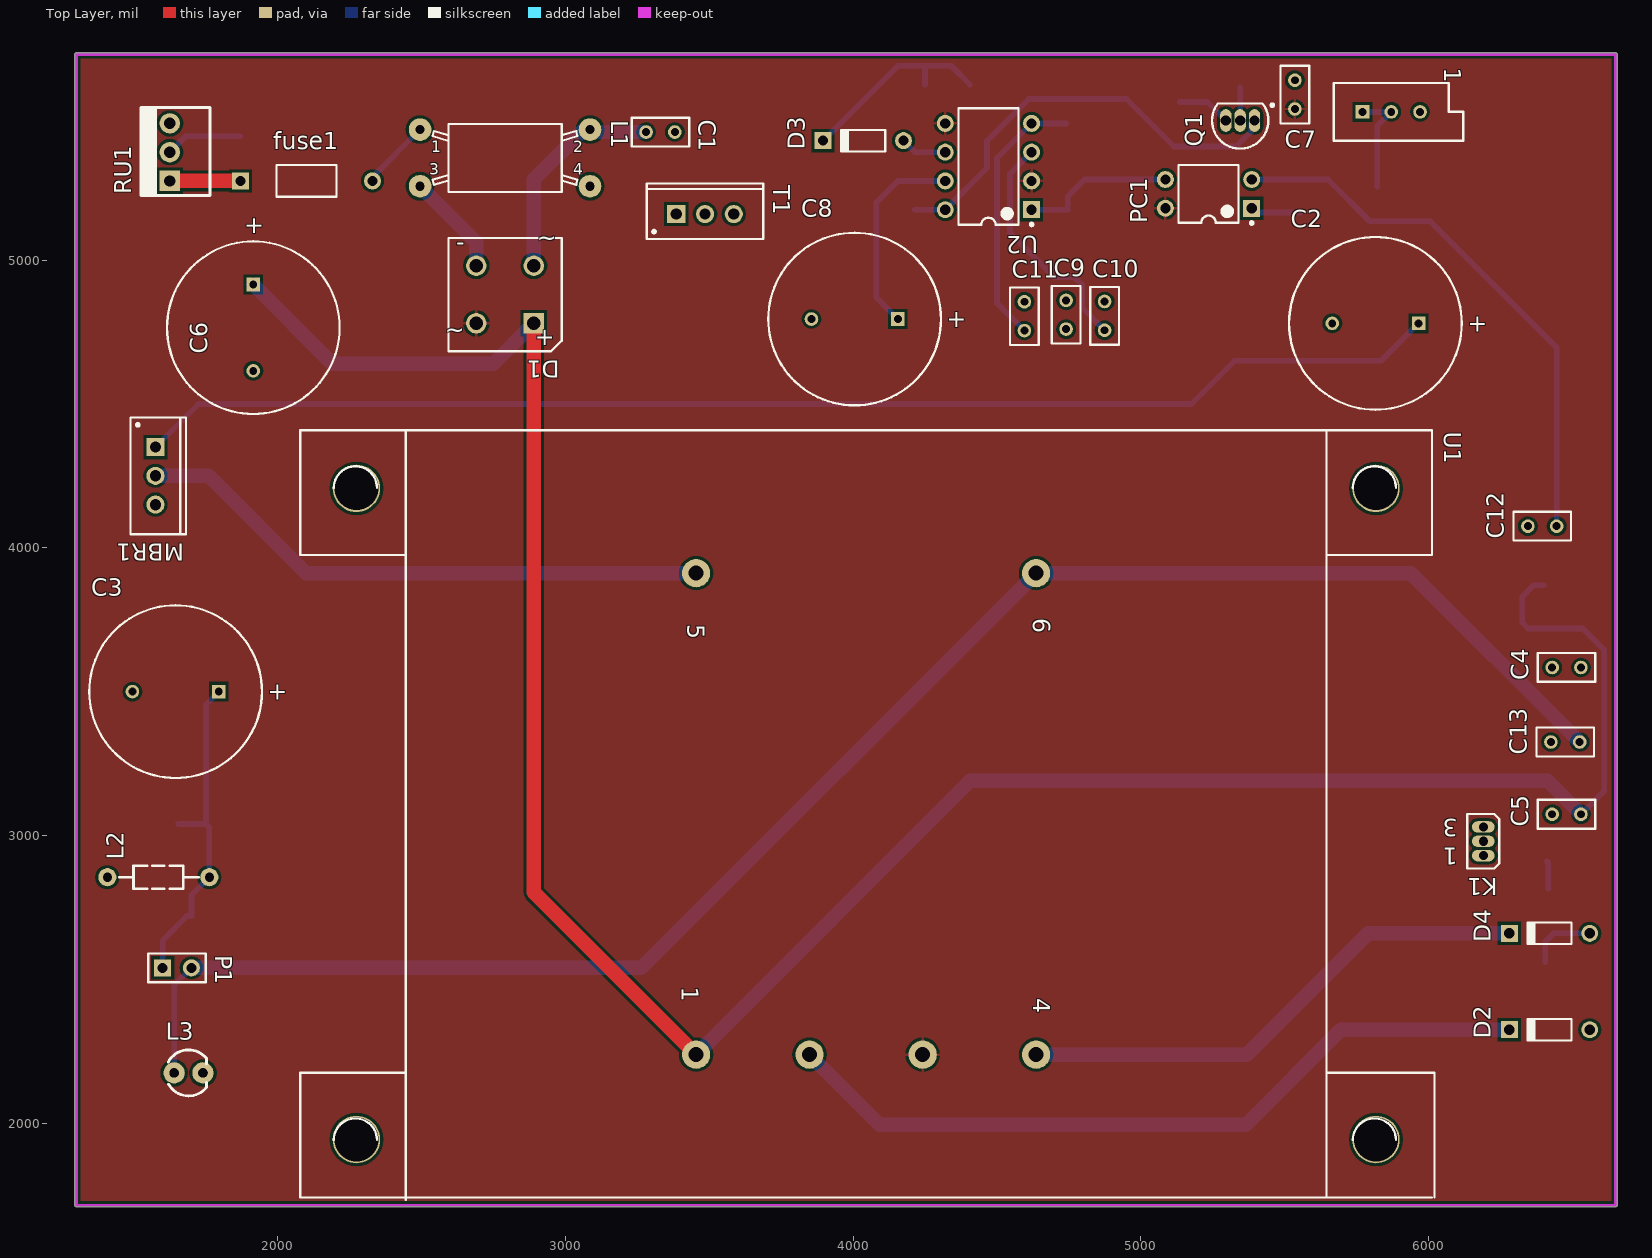
[diagram p0: Top Layer view]
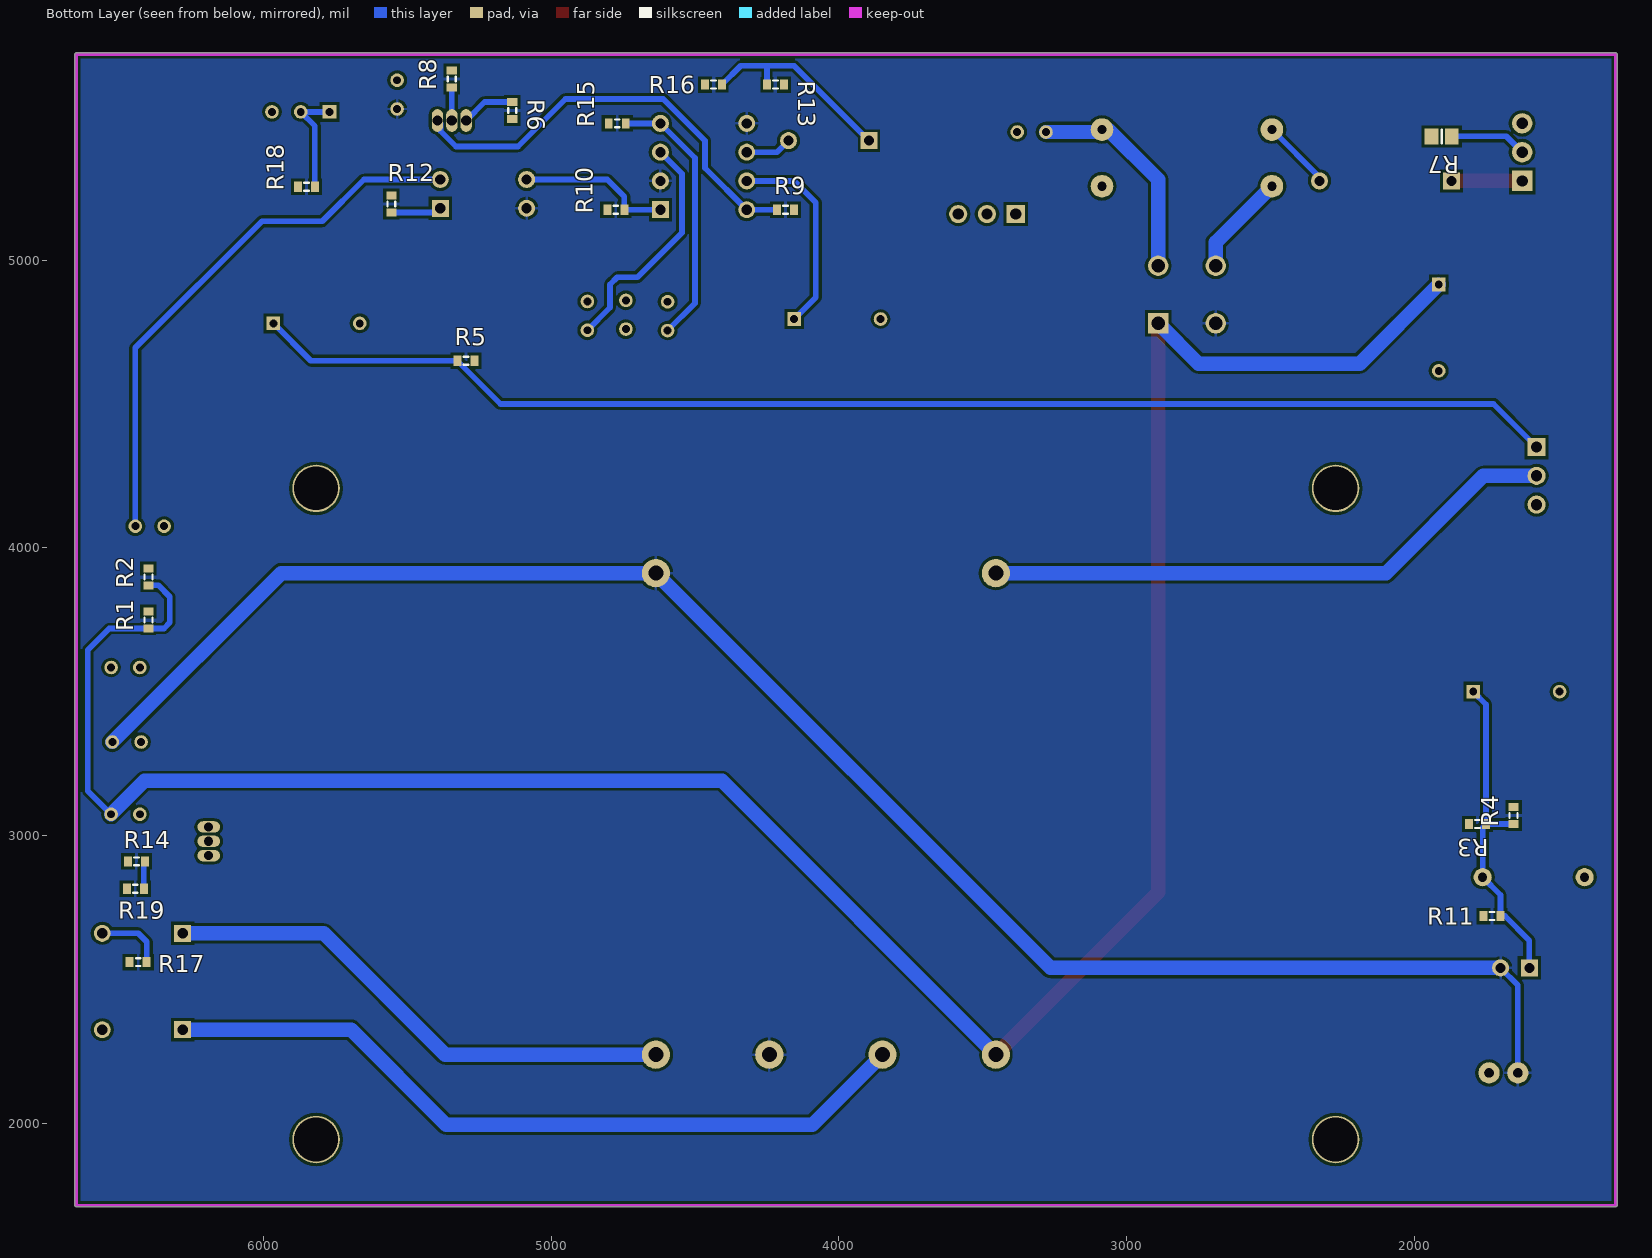
[diagram p1: Bottom Layer view, seen from below]
# Altium PCB MISC82118.PcbDoc
Units mil, origin at the board's own origin, x right, y up, seen from the top; angles counter-clockwise.
Board outline 5360.03 x 4010.03 mil, 2 copper layers (Top Layer, Bottom Layer); 50 components, 32 nets, 126 pads, 0 vias.

## Layer stack, top to bottom (the 12.6 mil dielectric is the usual default, probably not edited)
Top Solder: solder mask 0.4, Solder Resist, Dk 3.5
Top Layer: signal copper 1.4
Dielectric 1: dielectric 12.6, FR-4, Dk 4.8
Bottom Layer: signal copper 1.4
Bottom Solder: solder mask 0.4, Solder Resist, Dk 3.5

## Board outline
1300,1709.98 cw(c1300,1715) 1294.98,1715 1294.98,5715 cw(c1300,5715) 1300,5720.02 6650,5720.02 cw(c6650,5715) 6655.02,5715 6655.02,1715 cw(c6650,1715) 6650,1709.98

## Design rules (kind name [scope] priority, off if disabled: settings)
Clearance [All] p1: gap=10
MinimumSolderMaskSliver [All] p1: minsoldermaskwidth=0
PolygonConnect [All] p1: connectstyle=Relief reliefconductorwidth=10 reliefentries=4 polygonreliefangle="90 Angle" airgapwidth=10
RoutingVias [All] p1: holewidth=28 width=50 viastyle="Through Hole" minholewidth=28 minwidth=50 maxholewidth=28 maxwidth=50
SilkToSilkClearance [All] p1: silktosilkclearance=0
SilkToSolderMaskClearance [IsPad] p1: minsilkscreentomaskgap=0 clearancetoexposedcopper=TRUE
SolderMaskExpansion [All] p1: expansion=4
Width [All] p1: maxlimit=70 minlimit=10 preferedwidth=10
27 further rules are at their usual default settings.

## Components (designator, comment, footprint, x,y, rotation, side; value= is the part's Value field where it differs from the comment)
1 "" VR5 5870,5515 r0 top
C1 "0.1u 275V" RAD-0.1 3330,5445 r0 top
C2 "35V 1000U" RB7.6-15 5815,4780 r0 top
C3 "35V 1000U" RB7.6-15 1645,3500 r0 top
C4 "2KV 103" RAD-0.1 6479.33,3583.94 r180 top
C5 "222/2KV" RAD-0.1 6479.33,3073.94 r180 top
C6 "400V  82uF" RB7.6-15 1915,4765 r90 top
C7 "104" RAD-0.1 5535,5575 r90 top
C8 "35V100U" RB7.6-15 4005,4795 r0 top
C9 "225" RAD-0.1 4740,4810 r90 top
C10 "471" RAD-0.1 4873.77,4806.06 r90 top
C11 "222" RAD-0.1 4595,4805 r90 top
C12 "104" RAD-0.1 6395,4075 r180 top
C13 "104" RAD-0.1 6475,3325 r180 top
D1 "1N4007*4" D-38 2790,4880 r180 top
D2 "FR107" DO-35 6420,2325 r180 top
D3 "IN4148" DO-35 4035,5415 r180 top
D4 "FR107" DO-35 6420,2660 r180 top
fuse1 "" PIN-W2/E2.8 2100,5275 r0 top
K1 "20N60" E3 6190,2980 r180 top
L1 "Filter" TRANS 2790,5355 r0 top
L2 "100UH" AL0204 1585,2855 r180 top
L3 "LED" LED3MM 1690,2175 r0 top
MBR1 "" TO-262-AA 1575,4250 r270 top
P1 "Output" HDR1X2 1600,2540 r0 top
PC1 "*" DIP-4 5235,5230 r180 top
Q1 "S8550" TO-92A 5345,5485 r90 top
R1 "2W 150K" J1-0603 6399.33,3748.94 r90 bottom
R2 "2W 200K" J1-0603 6399.33,3898.94 r90 bottom
R3 "2W 330" J1-0603 1780,3040 r0 bottom
R4 "2K2" J1-0603 1655,3070 r90 bottom
R5 "10/1W" J1-0603 5295.47,4650 r180 bottom
R6 "68k" J1-0603 5135,5519.53 r270 bottom
R7 "NTC 5D-11" 6-0805_N 1904.57,5430 r0 bottom
R8 "4K1" J1-0603 5345,5629.53 r90 bottom
R9 "680" J1-0603 4185,5175 r180 bottom
R10 "4K1" J1-0603 4775,5175 r0 bottom
R11 "20K" J1-0603 1730,2720 r0 bottom
R12 "470" J1-0603 5555,5195 r90 bottom
R13 "15" J1-0603 4220.47,5610 r180 bottom
R14 "470" J1-0603 6440.47,2910 r0 bottom
R15 "18K" J1-0603 4770,5475 r0 bottom
R16 "1K" J1-0603 4435,5610 r0 bottom
R17 "1W 10" J1-0603 6435,2560 r0 bottom
R18 "2K2" J1-0603 5850.47,5255 r0 bottom
R19 "2W 0.62" J1-0603 6445,2815 r0 bottom
RU1 "*" KF2510-3P 1625,5275 r90 top
T1 "TL431" TO-262-AA 3485,5160 r0 top
U1 "Transformer 1" TRF_6 4045,3075 r270 top
U2 "UC3842" DIP-8 4470,5325 r180 top

## Footprints (in the part's own frame and the unit in brackets; to place one, negate y for a bottom-side part, rotate by r counter-clockwise, add the part's x,y. Pads: shape width x height; smd on the part's side, far side on the other; paste and mask are expansions set on the pad)
6-0805_N [mm] "Chip Resistor, Body 2.0x1.2mm, IPC Medium Density"
  rect 1.2x1.4 smd: 1(-0.9,0) 2(0.9,0)
  silkscreen extent 0,-0.6 0,0.6, body extent -1.07,-0.7 1.07,0.7, height 0.7
AL0204 [mm] "9*2*4mm（脚距，直径，长度）"
  round 1.6 hole 0.8: 1(-4.5,0) 2(4.5,0)
  silkscreen extent -3.56,-1.02 3.43,1.02, body extent -4.75,-1.02 4.75,1.02, height 2.07
D-38 [mm] "Bridge Rectifier; 4 Terminals; Body 9.4 x 9.4 mm (typ); Pitch 5.08 mm"
  rect 1.8x1.8 hole 1.2: 1(-2.54,2.54)
  round 1.8 hole 1.2: 2(-2.54,-2.54) 3(2.54,-2.54) 4(2.54,2.54)
  silkscreen extent -5,-5 5,5, body extent -5,-5 5,5, height 9.91
DIP-4 [mm] "DIP; 4 Leads; Row Spacing 7.62 mm; Pitch 2.54 mm"
  rect 1.5x1.5 hole 0.9: 1(-3.81,1.27)
  round 1.5 hole 0.9: 2(-3.81,-1.27) 3(3.81,-1.27) 4(3.81,1.27)
  silkscreen extent -3.94,-2.55 2.65,2.69, body extent -3.15,-2.5 3.15,2.5, height 5.6
DIP-8 [mm] "DIP; 8 Leads; Row Spacing 7.62 mm; Pitch 2.54 mm"
  rect 1.5x1.5 hole 0.9: 1(-3.81,3.81)
  round 1.5 hole 0.9: 2(-3.81,1.27) 3(-3.81,-1.27) 4(-3.81,-3.81) 5(3.81,-3.81) 6(3.81,-1.27) 7(3.81,1.27) 8(3.81,3.81)
  silkscreen extent -3.94,-5.15 2.65,5.23, body extent -3.6,-5.15 3.6,5.15, height 5.08
DO-35 [mm] "Diode, Axial; Body 3.8 x 1.9 mm (LxDia. max), Lead Dia. 0.53 mm (max)"
  round 1.5 hole 0.9: 1(-3.55,0)
  rect 1.5x1.5 hole 0.9: 2(3.55,0)
  silkscreen extent -1.95,-0.95 2.05,0.95
E3 [mm] "TO, Flat Index; 3 In-Line, Axial Leads; Body Dia. 4.6mm; Lead Dia. 0.5 mm (max)"
  oval 2x1 hole 0.8: 1(0,1.27) 2(0,0) 3(0,-1.27)
  silkscreen extent -1.41,-2.41 1.41,2.41
HDR1X2 [mm] "Connector; Header; 2 Position"
  rect 1.5x1.5 hole 0.9: 1(0,0)
  round 1.5 hole 0.9: 2(2.54,0)
  silkscreen extent -1.27,-1.27 3.81,1.27
J1-0603 [mm] "Chip Resistor, Body 1.6x0.8mm, IPC High Density"
  rect 0.7x0.9 smd: 1(-0.75,0) 2(0.75,0)
  silkscreen extent -0.2,-0.35 0.2,0.35, body extent -0.85,-0.48 0.85,0.48, height 0.9
KF2510-3P [mm]
  rect 1.8x1.8 hole 1: 1(0,0)
  round 1.8 hole 1: 2(2.54,0) 3(5.08,0)
  silkscreen extent -1.27,-3.56 6.48,2.54, body extent -1.27,-3.59 6.35,2.32, height 11.05
LED3MM [mil]
  round 74 hole 32 slot 32.2 at 0 deg paste+0 mask+2: 1(-50,0) 2(50,0)
  silkscreen extent -71,-80 62,80
PIN-W2/E2.8 [mm] "Thru-Hole; 2 Leads"
  rect 1.5x1.5 hole 0.9: 1(-5.825,0)
  round 1.5 hole 0.9: 2(5.825,0)
  silkscreen extent -2.65,-1.4 2.65,1.4
RAD-0.1 [mm] "Radial Cap, Thru-Hole; 2 Leads; 0.1 in Pin Spacing"
  round 1.2 hole 0.7: 1(-1.27,0) 2(1.27,0)
  silkscreen extent -2.54,-1.27 2.54,1.27
RB7.6-15 [mm] "Polarized Capacitor (Radial); 2 Leads"
  rect 1.2x1.2 hole 0.7: 1(3.81,0)
  round 1.2 hole 0.7: 2(-3.81,0)
  silkscreen extent -7.62,-7.62 7.62,7.62
TO-92A [mm] "TO, Flat Index; 3 In-Line, Axial Leads; Body Dia. 4.5mm; Leads 0.51 x 0.48 mm (max)"
  oval 2x1 hole 0.9: 1(0,-1.27) 2(0,0) 3(0,1.27)
  silkscreen extent -2.48,-2.96 1.5,2.48, body extent -2.48,-2.5 1.5,2.5, height 6.86
TO-262-AA [mm] "TO, Thru-Hole, Vertical, Heatsink Mounted; 3 In-Line Leads; Pitch 2.54 mm"
  rect 1.6x1.6 hole 1: 1(-2.54,0)
  round 1.6 hole 1: 2(0,0) 3(2.54,0)
  silkscreen extent -5.15,-2.2 5.15,2.7, body extent -5.2,-2.25 5.2,2.75, height 19.7
TRANS [mm] "Transformer; 4 Leads"
  round 2 hole 0.8: 1(-7.5,2.5) 2(7.5,2.5) 3(-7.5,-2.5) 4(7.5,-2.5)
  silkscreen extent -6.4,-3 6.4,3
TRF_6 [mil] "Transformer; 6 Leads"
  round 98 hole 52: 1(836.67,-590.83) 2(836.67,-196.67) 3(836.67,196.67) 4(836.67,590.83) 5(-836.67,-590.83) 6(-836.67,590.83)
  round 165 hole 152: MH1(-1131.67,-1771.67) MH2(1131.67,-1771.67) MH3(1131.67,1771.67) MH4(-1131.67,1771.67)
  silkscreen extent -1333,-1967 1342,1975
VR5 [mm] "Thru-Hole; 3 Leads"
  rect 1.2x1.2 hole 0.7: 1(-2.54,0)
  round 1.2 hole 0.7: 2(0,0) 3(2.54,0)
  silkscreen extent -5.08,-2.54 6.35,2.54

## Part data
1: library part 三角电位器
C1 C4 C5 C7 C9 C10 C11 C12 C13: library part 电容
C2 C3 C6 C8: library part 电解电容1
D1: library part BRIDGE1, "Diode Bridge"
D2 D4: library part 肖特基二极管
D3: library part 二极管
fuse1: library part 保险丝
K1: library part N-MOS
L1: library part 滤波器
L2: library part 电感
L3: library part 发光二极管
MBR1: library part 肖特基二极管2
P1: library part "Header 2", "Header, 2-Pin"
PC1: library part 光电耦合器
Q1: library part 2N3906, "PNP General Purpose Amplifier"
R1 R2 R3 R4 R5 R6 R7 R8 R9 R10 R11 R12 R13 R14 R15 R16 R17 R18 R19: library part 电阻
RU1: library part 接线端子3
U1: library part 变压器1

## Nets (pads, with @x,y where several pads share a name; then routed paths per layer and width w, separated by ;. In a path a pad name is that pad's centre, name@x,y a point inside that pad or via, vN(x,y) a via of type N, cw(c..) or ccw(c..) an arc to the next point about the centre after c; other vN are vias at no path point)
GND: C7.1 C13.1 D1.4 L3.1 P1.2 PC1.4 U1.3 U1.6 U2.2 U2.5 | length 6026
  Bottom Layer w20: L3.1 1640,2480 P1.2
  Bottom Layer w50: P1.2 3264.17,2540 U1.6 5938.33,3911.67 C13.1
Net1_1: 1.1 1.2 R18.1 | length 380.3
  Bottom Layer w20: 1.1 1.2 5820.94,5465.94 R18.1
NetC1_0: D1.3 L1.3 | length 357.5
  Bottom Layer w50: L1.3 2690,5061.3 D1.3
NetC1_1: C1.1 D1.2 L1.2 | length 765.3
  Bottom Layer w50: D1.2 2890,5280 3063.43,5453.43 L1.2 3093.7,5445 C1.1
NetC2_1: C2.1 MBR1.1 R5.1 | length 4568.5
  Bottom Layer w20: MBR1.1 1725,4500 5175.73,4500 5325,4649.27 R5.1 5835,4650 C2.1
NetC3_1: C3.1 L2.1 P1.1 R3.1 R4.1 R11.1 | length 1155.2
  Bottom Layer w20: P1.1 1600,2635 1685,2720 R11.1 1700.47,2793.31 L2.1 1762.17,3028.31 R3.1 ; R4.1 1655.47,3040 R3.1 ; C3.1 1750.47,3455.47 R3.1
NetC4_0: MBR1.2 U1.5 | length 2019.3
  Bottom Layer w50: MBR1.2 1760,4250 2098.33,3911.67 U1.5
NetC4_1: C4.1
NetC5_0: D2.1
NetC5_1: C5.1 C6.1 D1.1 R1.1 R2.1 U1.1 | length 8549.2
  Top Layer w50: D1.1 2890,2802.5 U1.1
  Bottom Layer w20: R2.1 6364.41,3869.41 6325,3830 6325,3740 6345.59,3719.41 R1.1 6535.59,3719.41 6610,3645 6610,3154.6 C5.1
  Bottom Layer w50: C6.1 2190,4640 2750,4640 D1.1 ; U1.1 4405.83,3190 6413.27,3190 C5.1
NetC7_0: Q1.1 R9.1 U2.8 | length 1516.3
  Bottom Layer w20: R9.1 U2.8 4465,5320 4465,5415 4610,5560 4950,5560 5115,5395 5330.81,5395 5384.69,5448.88 5384.69,5474.69 Q1.1
NetC8_1: C8.1 U2.7 | length 707.1
  Bottom Layer w20: C8.1 4080,4870 4080,5200 4155,5275 U2.7
NetC9_1: C9.1
NetC10_1: C10.1 U2.3 | length 827.2
  Bottom Layer w20: U2.3 4545,5300 4545,5095 4700,4940 4770,4940 4795,4915 4795,4834.83 C10.1
NetC11_1: C11.1 R15.1 U2.4 | length 929.5
  Bottom Layer w20: C11.1 4500,4850 4500,5355 U2.4 R15.1
NetC12_0: 
NetC12_1: C12.1 PC1.2 | length 1922.3
  Bottom Layer w20: PC1.2 5650,5280 5795,5135 6005,5135 6445,4695 C12.1
NetD2_2: D2.2 U1.2 | length 2669.4
  Bottom Layer w50: U1.2 4091.67,1995 5365,1995 5695,2325 D2.2
NetD3_1: D3.1 U2.6 | length 161.8
  Bottom Layer w20: D3.1 4214.76,5375 U2.6
NetD3_2: D3.2 R13.1 R16.1 | length 711.9
  Bottom Layer w20: D3.2 4155.24,5675 4245,5675 ; R13.1 4250,5670 4245,5675 ; R16.1 4340.47,5675 4245,5675
NetD4_1: D4.1 R17.1 | length 237
  Bottom Layer w20: R17.1 6405.47,2630.47 6435,2660 D4.1
NetD4_2: D4.2 U1.4 | length 1819.1
  Bottom Layer w50: U1.4 5368.33,2238.33 5790,2660 D4.2
Netfuse1_1: fuse1.1 RU1.1 | length 245.7
  Top Layer w50: RU1.1 fuse1.1
Netfuse1_2: fuse1.2 L1.1 | length 246.9
  Bottom Layer w20: fuse1.2 2329.33,5288.03 L1.1
NetK1_3S: R14.1 R19.1 | length 96.9
  Bottom Layer w20: R14.1 6415.47,2905.47 R19.1
NetL1_4: L1.4
NetL3_0: 
NetPC1_1: PC1.1 R12.1 | length 176
  Bottom Layer w20: PC1.1 5399.53,5165.47 R12.1
NetPC1_3: PC1.3 R10.1 U2.1 | length 535.1
  Bottom Layer w20: U2.1 R10.1 4745.47,5220.47 4805,5280 PC1.3
NetQ1_2: Q1.2 R8.1 | length 115
  Bottom Layer w20: Q1.2 R8.1
NetQ1_3: Q1.3 R6.1 | length 186.5
  Bottom Layer w20: R6.1 5230.94,5549.06 Q1.3
NetR7_1: R7.1 RU1.2 | length 266.9
  Bottom Layer w20: RU1.2 1680,5430 R7.1
pads on no net: 1.3 C1.2 C2.2 C3.2 C4.2 C5.2 C6.2 C7.2 C8.2 C9.2 C10.2 C11.2 C12.2 C13.2 K1.1 K1.2 K1.3 L2.2 L3.2 MBR1.3 R1.2 R2.2 R3.2 R4.2 R5.2 R6.2 R7.2 R8.2 R9.2 R10.2 R11.2 R12.2 R13.2 R14.2 R15.2 R16.2 R17.2 R18.2 R19.2 RU1.3 T1.1 T1.2 T1.3 U1.MH1 U1.MH2 U1.MH3 U1.MH4

## Polygon pours and split planes (outlines as drawn)
GND on Bottom Layer "G" (solid, remove dead copper, pour order 2): 765,5920 7020,5920 7055,5955 6975,5875 6975,1090 1250,1090 1020,1320
GND on Top Layer "G" (solid, remove dead copper, pour order 0): 605,6060 825,6280 7445,6280 7445,1480 7190,1225 6930,1485 785,1485

## Keep-outs
Keep-Out Layer:
  lines w10: 5745,1715 6650,1715 6650,5715 1300,5715 1300,1715 5765,1715